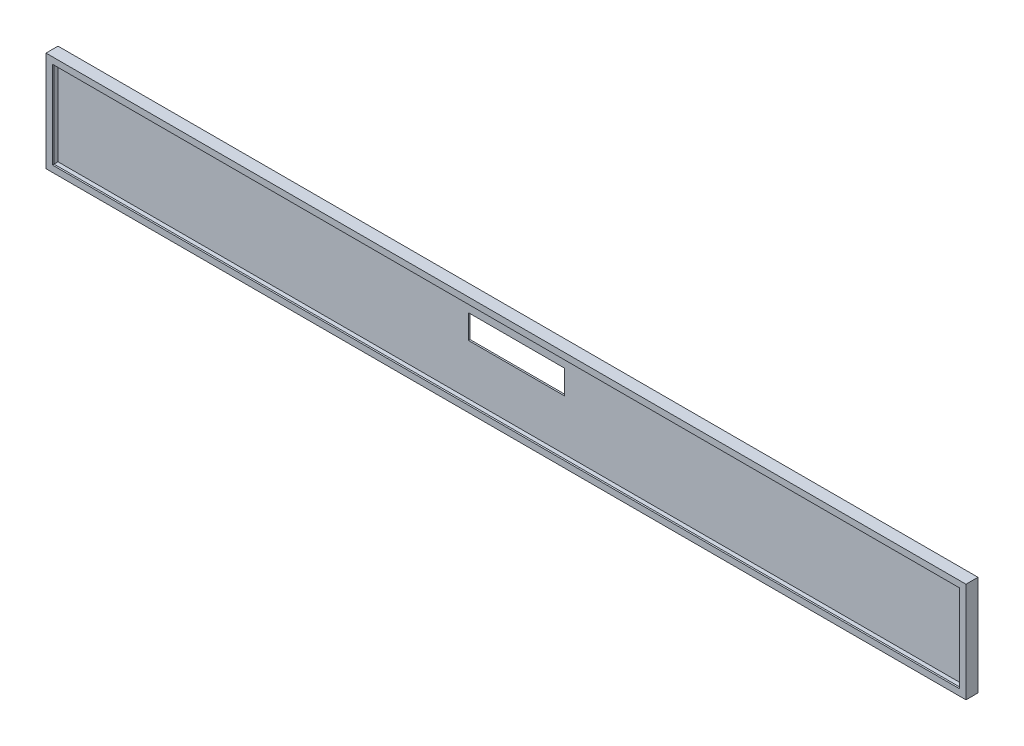
from build123d import *

# Parameters (mm, degrees)
SKETCH_1_W          = 1148
SKETCH_1_H          = 125
EXTRUDE_1_DEPTH     = 15
SHELL_1_T           = -2
SKETCH_2_W          = 1148
SKETCH_2_H          = 125
SKETCH_2_W_2        = 1132
SKETCH_2_H_2        = 109
EXTRUDE_2_DEPTH     = 2
SKETCH_3_W          = 120
SKETCH_3_H          = 30
CUT_EXTRUDE_1_DEPTH = 10


with BuildPart() as part:
    # 草图1 → 凸台-拉伸1 (new body)
    with BuildSketch(Plane.XY):
        with Locations((574, 62.5)):
            Rectangle(SKETCH_1_W, SKETCH_1_H)
    extrude(amount=EXTRUDE_1_DEPTH)

    # 抽壳1
    shell_1_openings = [part.faces().sort_by_distance(p)[0] for p in [
        (574, 62.5, 15),
    ]]
    offset(amount=SHELL_1_T, openings=shell_1_openings, kind=Kind.INTERSECTION)

    # 草图2 → 凸台-拉伸2 (add)
    with BuildSketch(Plane.XY.offset(15)):
        with Locations((574, 62.5)):
            Rectangle(SKETCH_2_W, SKETCH_2_H)
        with Locations((574, 62.5)):
            Rectangle(SKETCH_2_W_2, SKETCH_2_H_2, mode=Mode.SUBTRACT)
    extrude(amount=-EXTRUDE_2_DEPTH)

    # 草图3 → 切除-拉伸1 (cut)
    with BuildSketch(Plane(origin=(0, 0, 0), x_dir=(-1, 0, 0), z_dir=(0, 0, -1))):
        with Locations((-574, 80)):
            Rectangle(SKETCH_3_W, SKETCH_3_H)
    extrude(amount=-CUT_EXTRUDE_1_DEPTH, mode=Mode.SUBTRACT)


solid = part.part
